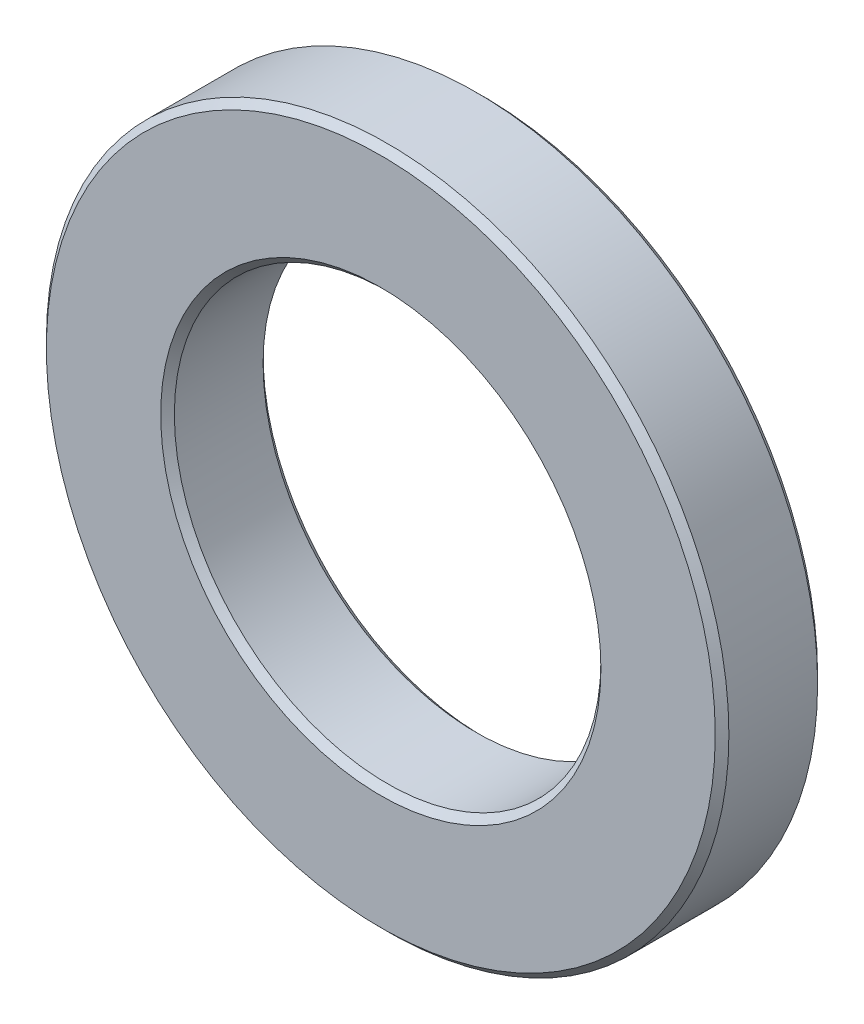
from build123d import *

# Parameters (mm, degrees)
SKETCH1_R           = 10
SKETCH1_R_2         = 6.25
BOSS_EXTRUDE1_DEPTH = 3
CHAMFER1_SIZE       = 0.2


with BuildPart() as part:
    # Sketch1 → Boss-Extrude1 (new body)
    with BuildSketch(Plane.XY):
        Circle(SKETCH1_R)
        Circle(SKETCH1_R_2, mode=Mode.SUBTRACT)
    extrude(amount=BOSS_EXTRUDE1_DEPTH)

    # Chamfer1
    chamfer1_edges = [part.edges().sort_by_distance(p)[0] for p in [
        (-10, 0, 0),
        (-10, 0, 3),
        (-6.25, 0, 0),
        (-6.25, 0, 3),
    ]]
    chamfer(chamfer1_edges, length=CHAMFER1_SIZE)


solid = part.part
